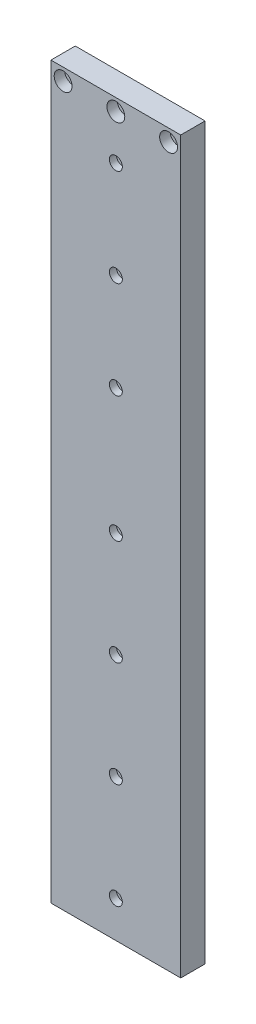
SolidWorks part; units mm, degrees
ref_plane "前视基准面" through (0, 0, 0) normal (0, 0, 1) x (1, 0, 0)
ref_plane "上视基准面" through (0, 0, 0) normal (0, 1, 0) x (1, 0, 0)
ref_plane "右视基准面" through (0, 0, 0) normal (1, 0, 0) x (0, 0, -1)
sketch "草图1" plane through (0, 0, 0) normal (0, 0, 1) x (1, 0, 0)
  line L1 (-40, -225) -> (40, -225)
  line L2 (-40, -225) -> (-40, 225)
  line L3 (-40, 225) -> (40, 225)
  line L4 (40, -225) -> (40, 225)
  line L5 (-40, -225) -> (40, 225) construction
  line L6 (-40, 225) -> (40, -225) construction
  point P0 (0, 0)
  dimension "D1" = 450
  dimension "D2" = 80
extrude "凸台-拉伸1" add sketch "草图1" along normal blind 15
hole_wizard "M6 六角凹头螺钉的柱形沉头孔1" positions "草图3" profile "草图4" counterbore size "M6" standard "ISO" end condition through all
sketch "草图3" plane through (0, 0, 15) normal (0, 0, 1) x (1, 0, 0)
  line L0 (0, 223) -> (0, 80.4222) construction
  line L3 (40, 225) -> (-40, 225) construction
  point P0 (-32.5, 217.5)
  point P2 (32.5, 217.5)
  point P35 (0, 217.5)
  dimension "D1" = 65
  dimension "D3" = 7.5
sketch "草图4" plane through (-32.5, 217.5, 15) normal (1, 0, 0) x (0, -1, 0)
  line L0 (0, 0) -> (0, 15)
  line L1 (0, 15) -> (3.3, 15)
  line L3 (3.3, 15) -> (3.3, 6.4)
  line L4 (3.3, 6.4) -> (5.5, 6.4)
  line L5 (5.5, 6.4) -> (5.5, 0)
  line L7 (5.5, 0) -> (0, 0)
  line L11 (0, -6.35) -> (0, 107.95) construction
  dimension "通孔孔直径" = 6.6
  dimension "通孔孔深度" = 15
  dimension "柱形沉头孔直径" = 11
  dimension "柱形沉头孔深度" = 6.4
hole_wizard "M4 六角凹头螺钉的柱形沉头孔1" positions "草图5" profile "草图6" counterbore size "M4" standard "ISO" end condition through all
sketch "草图5" plane through (0, 0, 15) normal (0, 0, 1) x (1, 0, 0)
  line L0 (0, 225) -> (0, 0) construction
  line L1 (40, 225) -> (-40, 225) construction
  point P0 (0, 190)
  point P2 (0, 130)
  point P4 (0, 70)
  dimension "D1" = 35
  dimension "D2" = 60
  dimension "D3" = 60
sketch "草图6" plane through (0, 190, 15) normal (1, 0, 0) x (0, -1, 0)
  line L0 (0, 0) -> (0, 15)
  line L1 (0, 15) -> (2.25, 15)
  line L3 (2.25, 15) -> (2.25, 4.4)
  line L4 (2.25, 4.4) -> (4, 4.4)
  line L5 (4, 4.4) -> (4, 0)
  line L7 (4, 0) -> (0, 0)
  line L11 (0, -6.35) -> (0, 107.95) construction
  dimension "通孔孔直径" = 4.5
  dimension "通孔孔深度" = 15
  dimension "柱形沉头孔直径" = 8
  dimension "柱形沉头孔深度" = 4.4
hole_wizard "M4 六角凹头螺钉的柱形沉头孔2" positions "草图7" profile "草图8" counterbore size "M4" standard "ISO" end condition through all
sketch "草图7" plane through (0, 0, 15) normal (0, 0, 1) x (1, 0, 0)
  line L0 (0, -225) -> (0, 0) construction
  line L1 (-40, -225) -> (40, -225) construction
  point P0 (0, -202.5)
  point P2 (0, -137.5)
  point P4 (0, -72.5)
  point P6 (0, -7.5)
  dimension "D1" = 22.5
  dimension "D2" = 65
  dimension "D3" = 65
  dimension "D4" = 65
sketch "草图8" plane through (0, -202.5, 15) normal (1, 0, 0) x (0, -1, 0)
  line L0 (0, 0) -> (0, 15)
  line L1 (0, 15) -> (2.25, 15)
  line L3 (2.25, 15) -> (2.25, 4.4)
  line L4 (2.25, 4.4) -> (4, 4.4)
  line L5 (4, 4.4) -> (4, 0)
  line L7 (4, 0) -> (0, 0)
  line L11 (0, -6.35) -> (0, 107.95) construction
  dimension "通孔孔直径" = 4.5
  dimension "通孔孔深度" = 15
  dimension "柱形沉头孔直径" = 8
  dimension "柱形沉头孔深度" = 4.4
hole_wizard "M6 螺纹孔1" positions "草图9" profile "草图10" tap size "M6" standard "ISO"
sketch "草图9" plane through (0, -225, 0) normal (0, -1, 0) x (-1, 0, 0)
  line L0 (40, -7.5) -> (-40, -7.5) construction
  line L1 (40, -15) -> (40, 0) construction
  line L2 (-40, -15) -> (-40, 0) construction
  line L4 (0, -15) -> (0, 0) construction
  line L5 (40, -15) -> (-40, -15) construction
  point P0 (32.5, -7.5)
  point P2 (0, -7.5)
  point P4 (-32.5, -7.5)
  dimension "D1" = 65
sketch "草图10" plane through (-32.5, -225, 7.5) normal (1, 0, 0) x (0, 0, -1)
  line L0 (0, 0) -> (0, 16.5022)
  line L1 (0, 16.5022) -> (2.5, 15)
  line L2 (2.5, 15) -> (2.5, 0)
  line L5 (2.5, 0) -> (0, 0)
  line L10 (0, 16.5022) -> (-2.5, 15) construction
  line L11 (0, -6.35) -> (0, 107.95) construction
  dimension "螺纹孔钻头直径" = 5
  dimension "螺纹孔钻头深度" = 15
  dimension "导头角度" = 118
cosmetic thread "孔螺蚊线1" parameters "D1"=14, "D2"=6
cosmetic thread "孔螺蚊线2" parameters "D1"=14, "D2"=6
cosmetic thread "孔螺蚊线3" parameters "D1"=14, "D2"=6
